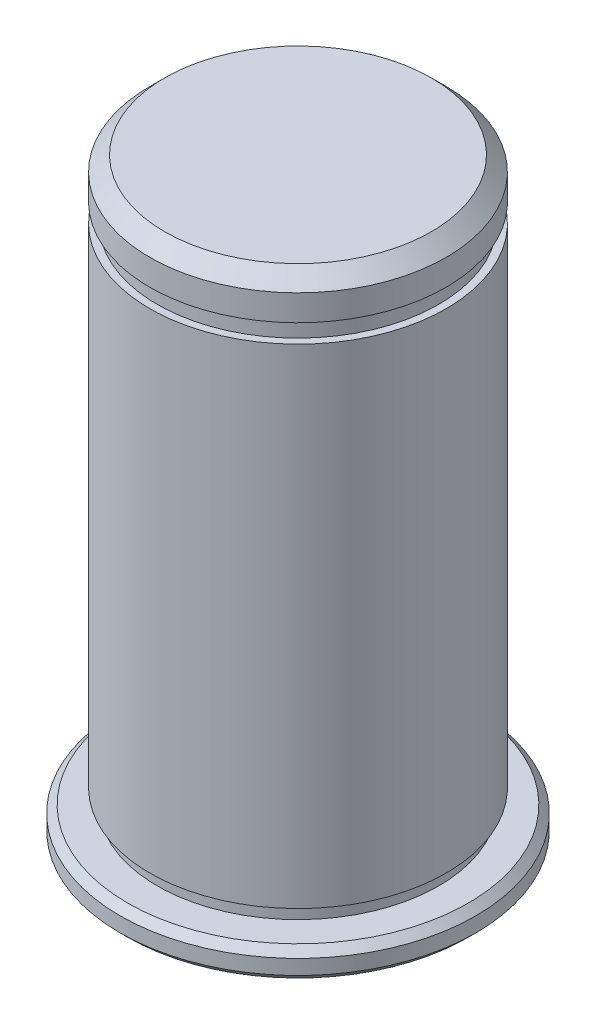
SolidWorks part; units mm, degrees
material "S45C"
ref_plane "前视基准面" through (0, 0, 0) normal (0, 0, 1) x (1, 0, 0)
ref_plane "上视基准面" through (0, 0, 0) normal (0, 1, 0) x (1, 0, 0)
ref_plane "右视基准面" through (0, 0, 0) normal (1, 0, 0) x (0, 0, -1)
sketch "草图1" plane through (0, 0, 0) normal (0, 0, 1) x (1, 0, 0)
  line L0 (0, -1.4673) -> (0, 33.274) construction
  line L1 (11.5, 2) -> (9.5, 2)
  line L2 (0, 0) -> (11.5, 0)
  line L3 (0, 0) -> (0, 40)
  line L4 (0, 40) -> (9, 40)
  line L5 (12, 0.5) -> (12, 1.5)
  line L6 (9.5, 2) -> (9.5, 3)
  line L7 (9.5, 3) -> (10, 3)
  line L8 (10, 3) -> (10, 36)
  line L9 (10, 37.25) -> (9.5, 37.25)
  line L10 (9.5, 37.25) -> (9.5, 36)
  line L11 (9.5, 36) -> (10, 36)
  line L12 (10, 37.25) -> (10, 39)
  line L13 (12, 1.5) -> (11.5, 2)
  line L14 (11.5, 0) -> (12, 0.5)
  line L15 (10, 39) -> (9, 40)
  point P6 (12, 0)
  point P7 (12, 2)
  point P12 (10, 40)
  dimension "D1" = 24
  dimension "D2" = 2
  dimension "D3" = 1
  dimension "D4" = 19
  dimension "D5" = 40
  dimension "D6" = 20
  dimension "D7" = 34
  dimension "D8" = 19
  dimension "D9" = 1.25
revolve "旋转1" add sketch "草图1" angle 360 about L0
